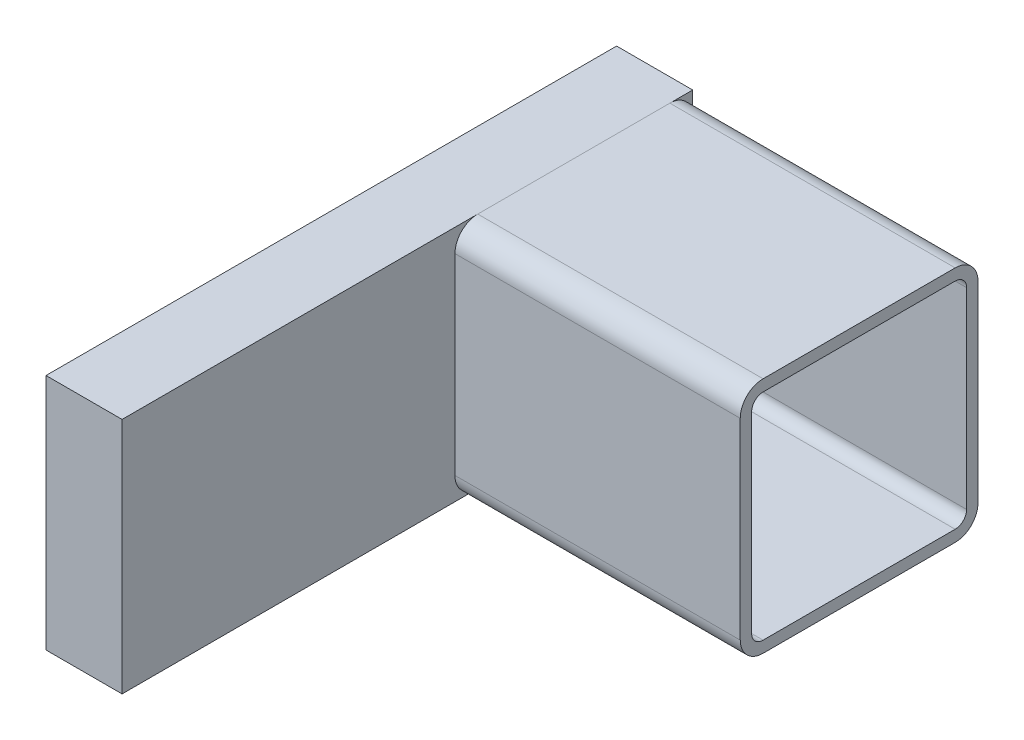
from build123d import *

# Parameters (mm, degrees)
GB_6728_1986_SQUARE_HOLLOW_SECTION_025_X_DEPTH = 30
SKETCH3_W                                      = 60
SKETCH3_H                                      = 25
BOSS_EXTRUDE1_DEPTH                            = 8


with BuildPart() as part:
    # Sketch1 → Gb／6728-1986 square hollow section 025 X 25 X 1.2(1) (new body)
    with BuildSketch(Plane(origin=(-15, 0, 0), x_dir=(0, 0, -1), z_dir=(1, 0, 0))):
        with BuildLine():
            Line((-10.1, -12.5), (10.1, -12.5))
            ThreePointArc((10.1, -12.5), (11.797056275, -11.797056275), (12.5, -10.1))
            Line((12.5, -10.1), (12.5, 10.1))
            ThreePointArc((12.5, 10.1), (11.797056275, 11.797056275), (10.1, 12.5))
            Line((10.1, 12.5), (-10.1, 12.5))
            ThreePointArc((-10.1, 12.5), (-11.797056275, 11.797056275), (-12.5, 10.1))
            Line((-12.5, 10.1), (-12.5, -10.1))
            ThreePointArc((-12.5, -10.1), (-11.797056275, -11.797056275), (-10.1, -12.5))
        make_face()
        with BuildLine():
            Line((-10.1, -11.3), (10.1, -11.3))
            ThreePointArc((10.1, -11.3), (10.948528137, -10.948528137), (11.3, -10.1))
            Line((11.3, -10.1), (11.3, 10.1))
            ThreePointArc((11.3, 10.1), (10.948528137, 10.948528137), (10.1, 11.3))
            Line((10.1, 11.3), (-10.1, 11.3))
            ThreePointArc((-10.1, 11.3), (-10.948528137, 10.948528137), (-11.3, 10.1))
            Line((-11.3, 10.1), (-11.3, -10.1))
            ThreePointArc((-11.3, -10.1), (-10.948528137, -10.948528137), (-10.1, -11.3))
        make_face(mode=Mode.SUBTRACT)
    extrude(amount=GB_6728_1986_SQUARE_HOLLOW_SECTION_025_X_DEPTH)


with BuildPart() as body_2:
    # Sketch3 → Boss-Extrude1 (new body)
    with BuildSketch(Plane.ZY.offset(15)):
        with Locations((17.5, 0)):
            Rectangle(SKETCH3_W, SKETCH3_H)
    extrude(amount=BOSS_EXTRUDE1_DEPTH)


solid = Compound([part.part, body_2.part])
